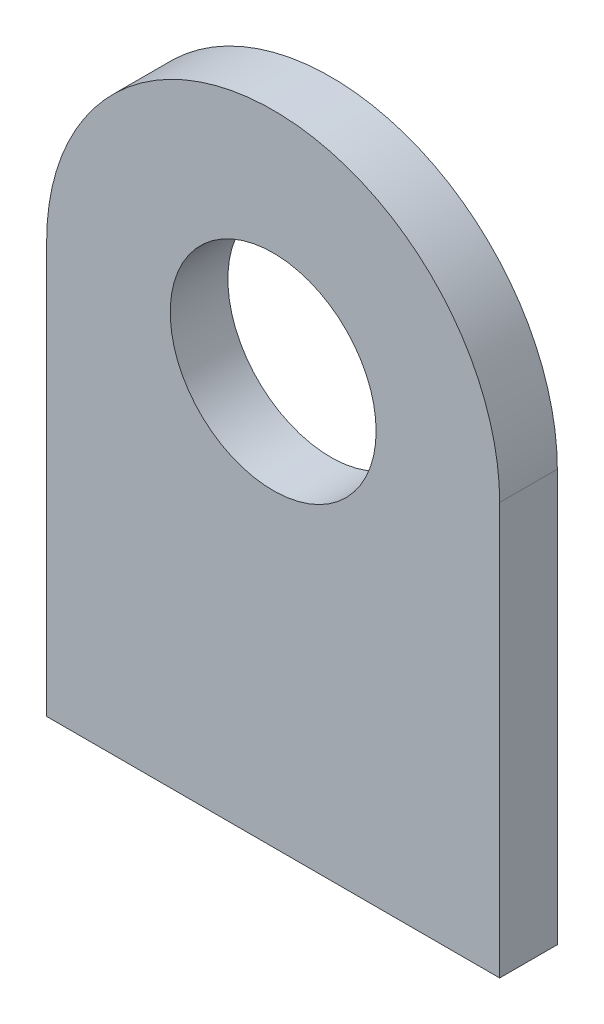
from build123d import *

# Parameters (mm, degrees)
SKETCH1_R           = 25
BOSS_EXTRUDE1_DEPTH = 14


with BuildPart() as part:
    # Sketch1 → Boss-Extrude1 (new body)
    with BuildSketch(Plane.XY):
        with BuildLine():
            Line((-55, 0), (-55, -100))
            Line((-55, -100), (55, -100))
            Line((55, -100), (55, 0))
            ThreePointArc((55, 0), (0, 55), (-55, 0))
        make_face()
        Circle(SKETCH1_R, mode=Mode.SUBTRACT)
    extrude(amount=BOSS_EXTRUDE1_DEPTH)


solid = part.part
